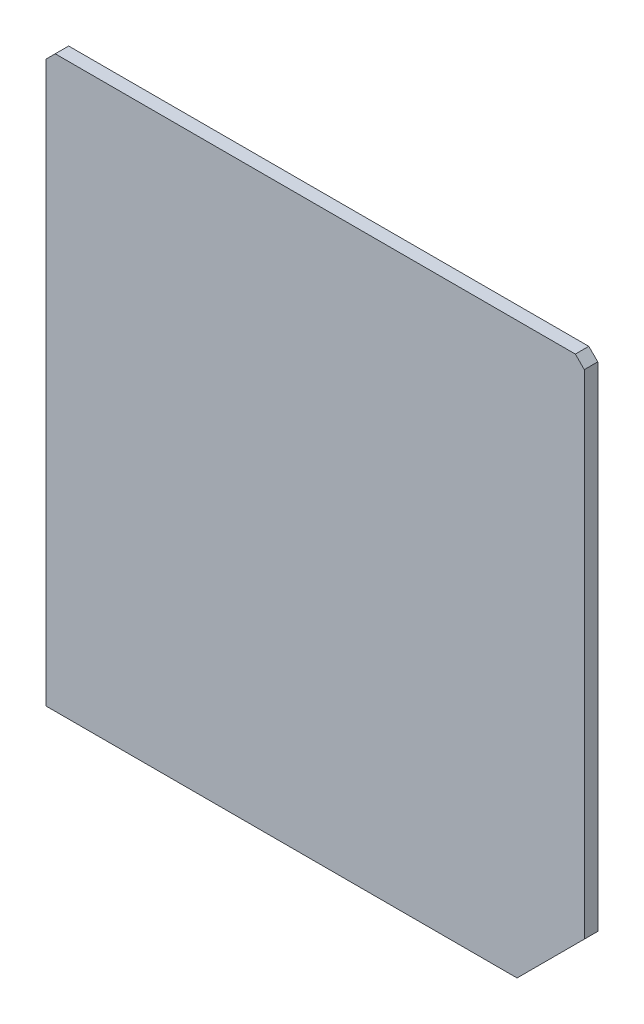
from build123d import *

# Parameters (mm, degrees)
SKETCH1_W           = 120
SKETCH1_H           = 127
BOSS_EXTRUDE1_DEPTH = 3
CHAMFER1_SIZE       = 15
CHAMFER2_SIZE       = 2


with BuildPart() as part:
    # Sketch1 → Boss-Extrude1 (new body)
    with BuildSketch(Plane.XY):
        Rectangle(SKETCH1_W, SKETCH1_H)
    extrude(amount=BOSS_EXTRUDE1_DEPTH)

    # Chamfer1
    chamfer1_edges = [part.edges().sort_by_distance(p)[0] for p in [
        (60, -63.5, 1.5),
    ]]
    chamfer(chamfer1_edges, length=CHAMFER1_SIZE)

    # Chamfer2
    chamfer2_edges = [part.edges().sort_by_distance(p)[0] for p in [
        (-60, 63.5, 1.5),
        (60, 63.5, 1.5),
    ]]
    chamfer(chamfer2_edges, length=CHAMFER2_SIZE)


solid = part.part
